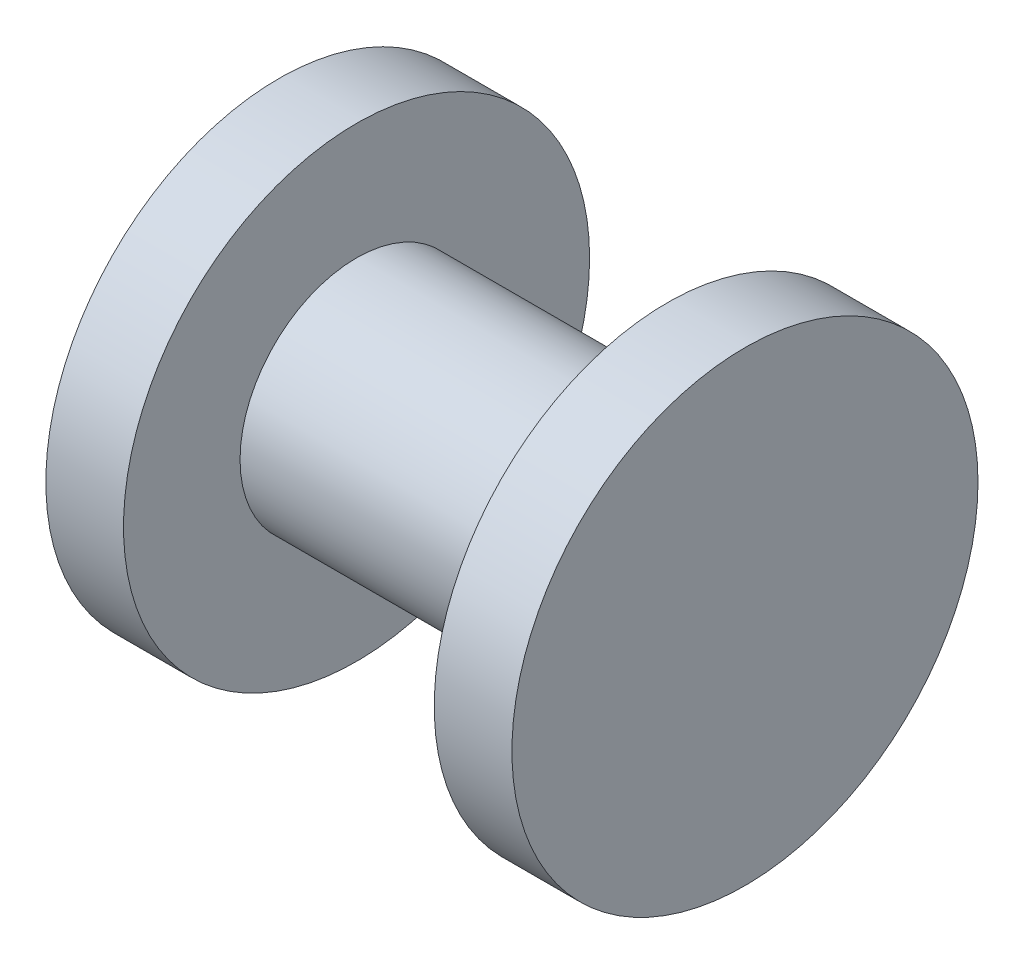
from build123d import *

# Parameters (mm, degrees)
SCALE1_SCALE = 0.3


with BuildPart() as part:
    # Sketch2 → Revolve1 (revolve)
    with BuildSketch(Plane.XY, mode=Mode.PRIVATE) as revolve1_sk:
        Polygon((10, -7.5), (10, -15), (15, -15), (15, 0), (-15, 0), (-15, -15), (-10, -15), (-10, -7.5), align=None)
    revolve(revolve1_sk.sketch.rotate(Axis((15, 0, 0), (-1, 0, 0)), 270), axis=Axis((15, 0, 0), (-1, 0, 0)))


with BuildPart() as part_1:
    # Scale1: scaled about (0, 0, 0)
    add(part.part.scale(SCALE1_SCALE))


solid = part_1.part
